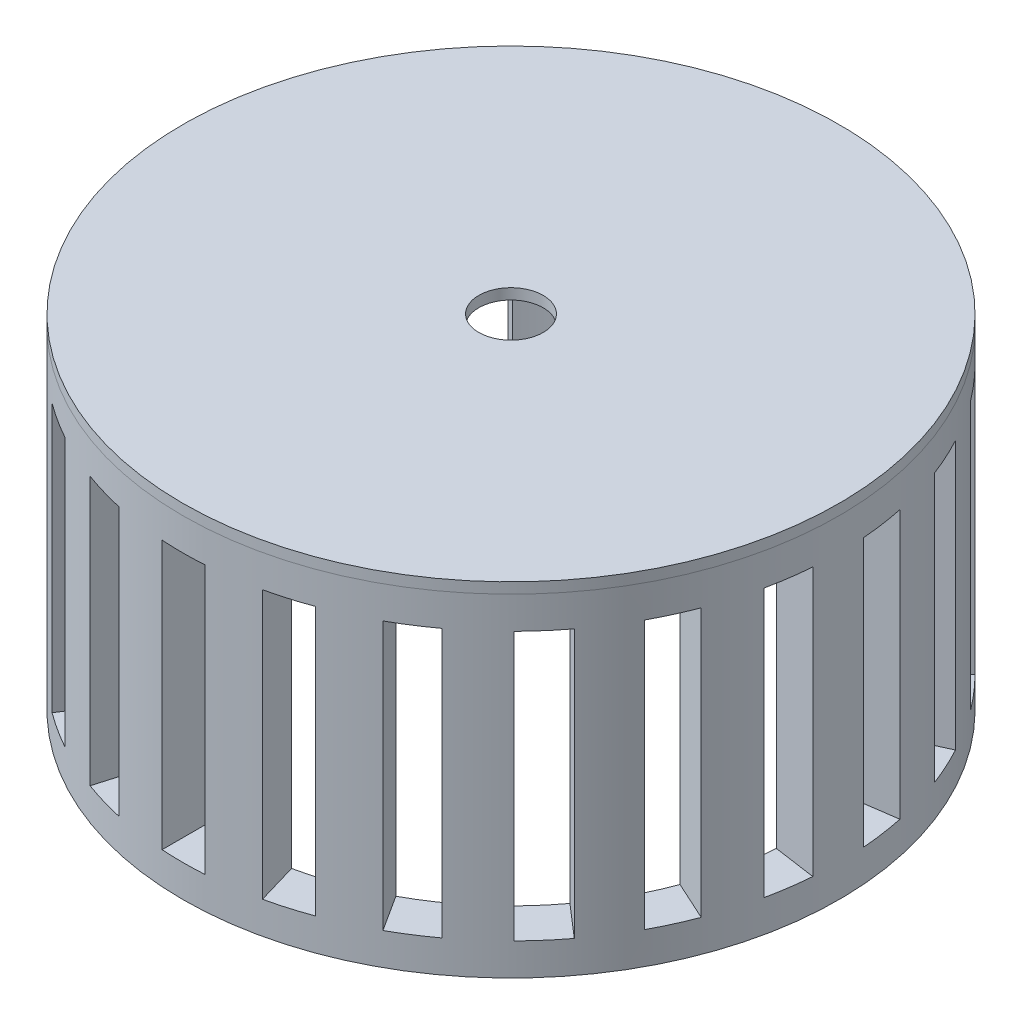
from build123d import *

# Parameters (mm, degrees)
SKETCH1_R           = 153
SKETCH1_R_2         = 133
BOSS_EXTRUDE1_DEPTH = 155
SKETCH2_W           = 20
SKETCH2_H           = 125
CUT_EXTRUDE1_DEPTH  = 267.163483596
CIRPATTERN1_COUNT   = 22
SKETCH3_R           = 153
BOSS_EXTRUDE2_DEPTH = 5
SKETCH4_R           = 15
CUT_EXTRUDE2_DEPTH  = 270.105927099


with BuildPart() as part:
    # Sketch1 → Boss-Extrude1 (new body)
    with BuildSketch(Plane(origin=(0, 0, 0), x_dir=(1, 0, 0), z_dir=(0, 1, 0))):
        with Locations(Location((0, 0, 0), (0, 0, 270))):
            Circle(SKETCH1_R)
        with Locations(Location((0, 0, 0), (0, 0, 270))):
            Circle(SKETCH1_R_2, mode=Mode.SUBTRACT)
    extrude(amount=BOSS_EXTRUDE1_DEPTH)

    # Sketch2 → Cut-Extrude1 (cut, symmetric)
    with BuildSketch(Plane.XY):
        with Locations((0, 77.5)):
            Rectangle(SKETCH2_W, SKETCH2_H)
    cut_extrude1 = extrude(amount=CUT_EXTRUDE1_DEPTH, both=True, mode=Mode.SUBTRACT)

    # CirPattern1: Cut-Extrude1 ×22 about axis
    cirpattern1_axis = Axis((0, 0, 0), (0, 1, 0))
    for i in range(1, CIRPATTERN1_COUNT):
        add(cut_extrude1.rotate(cirpattern1_axis, i * 360 / CIRPATTERN1_COUNT), mode=Mode.SUBTRACT)


with BuildPart() as body_2:
    # Sketch3 → Boss-Extrude2 (new body)
    with BuildSketch(Plane(origin=(0, 155, 0), x_dir=(1, 0, 0), z_dir=(0, 1, 0))):
        with Locations(Location((0, 0, 0), (0, 0, 270))):
            Circle(SKETCH3_R)
    extrude(amount=BOSS_EXTRUDE2_DEPTH)

    # Sketch4 → Cut-Extrude2 (cut, through all)
    with BuildSketch(Plane(origin=(0, 160, 0), x_dir=(1, 0, 0), z_dir=(0, 1, 0))):
        with Locations(Location((0, 0, 0), (0, 0, 270))):
            Circle(SKETCH4_R)
    extrude(amount=-CUT_EXTRUDE2_DEPTH, mode=Mode.SUBTRACT)


solid = Compound([part.part, body_2.part])
